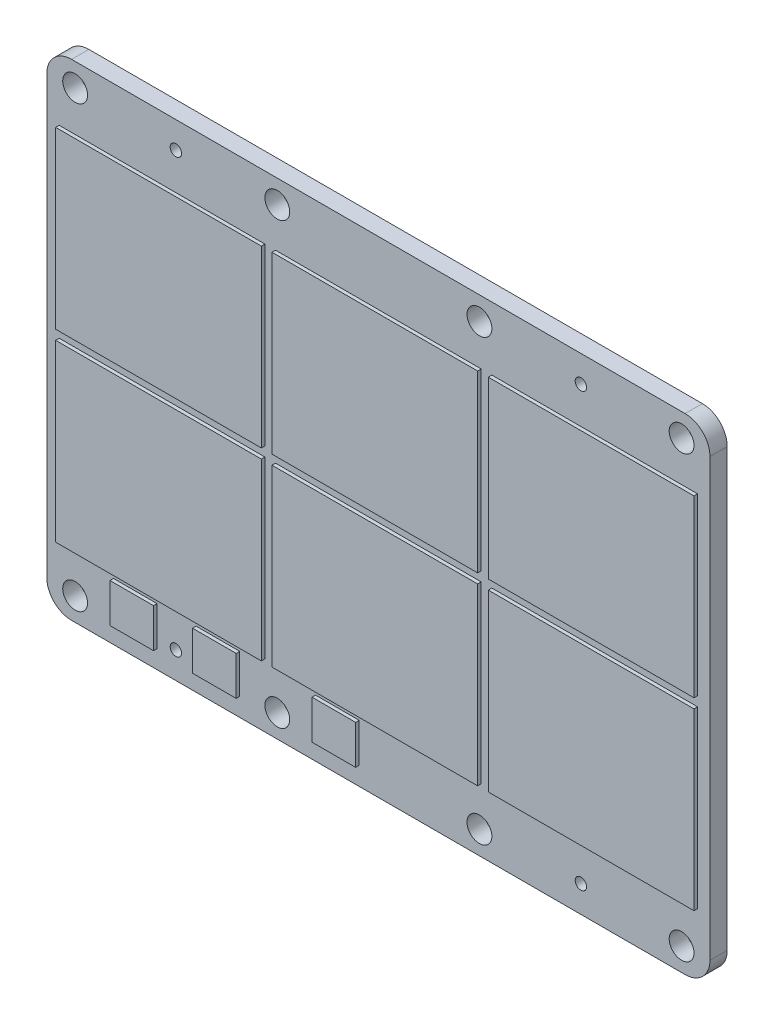
SolidWorks part; units mm, degrees
ref_plane "Front Plane" through (0, 0, 0) normal (0, 0, 1) x (1, 0, 0)
ref_plane "Top Plane" through (0, 0, 0) normal (0, 1, 0) x (1, 0, 0)
ref_plane "Right Plane" through (0, 0, 0) normal (1, 0, 0) x (0, 0, -1)
sketch "Sketch1" plane through (0, 0, 0) normal (0, 0, 1) x (1, 0, 0)
  line L1 (-93.5, 68.5) -> (93.5, 68.5)
  line L2 (-93.5, 68.5) -> (-93.5, -68.5)
  line L3 (-93.5, -68.5) -> (93.5, -68.5)
  line L4 (93.5, 68.5) -> (93.5, -68.5)
  line L5 (-93.5, 68.5) -> (93.5, -68.5) construction
  line L6 (-93.5, -68.5) -> (93.5, 68.5) construction
  point P0 (0, 0)
  dimension "D1" = 187
  dimension "D2" = 137
extrude "Boss-Extrude1" add sketch "Sketch1" along normal blind 4.87
hole_wizard "Ø7.0 (7) Diameter Hole1" positions "Sketch3" profile "Sketch2" hole size "Ø7.0" standard "ISO" end condition through all
sketch "Sketch3" plane through (0, 0, 4.87) normal (0, 0, 1) x (1, 0, 0)
  line L0 (-93.5, 68.5) -> (-93.5, -68.5) construction
  line L1 (0, 0) -> (-28.5, 0) construction
  point P0 (-28.5, 62)
  point P1 (-85.5, 62)
  point P3 (28.5, 62)
  point P9 (85.5, 62)
  point P19 (85.5, -62)
  point P20 (28.5, -62)
  point P21 (-85.5, -62)
  point P22 (-28.5, -62)
  dimension "D1" = 57
  dimension "D2" = 57
  dimension "D3" = 57
  dimension "D4" = 8
  dimension "D5" = 62
sketch "Sketch2" plane through (-28.5, 62, 4.87) normal (1, 0, 0) x (0, -1, 0)
  line L0 (0, 0) -> (0, 4.87)
  line L1 (0, 4.87) -> (3.5, 4.87)
  line L2 (3.5, 4.87) -> (3.5, 0)
  line L5 (3.5, 0) -> (0, 0)
  line L11 (0, -6.35) -> (0, 107.95) construction
  dimension "通孔孔直径" = 7
  dimension "通孔孔深度" = 4.87
hole_wizard "Ø3.2 (3.2) Diameter Hole1" positions "Sketch4" profile "Sketch5" hole size "Ø3.2" standard "ISO" end condition through all
sketch "Sketch4" plane through (0, 0, 4.87) normal (0, 0, 1) x (1, 0, 0)
  line L1 (0, 0) -> (30.398, 0) construction
  line L3 (-93.5, 68.5) -> (-93.5, -68.5) construction
  point P0 (-57.1, 61.02)
  point P2 (57.1, 60.975)
  point P4 (57.1, -60.975)
  point P6 (-57.1, -61.02)
  dimension "D1" = 121.95
  dimension "D2" = 122.04
  dimension "D3" = 36.4
  dimension "D4" = 114.2
sketch "Sketch5" plane through (-57.1, 61.02, 4.87) normal (1, 0, 0) x (0, -1, 0)
  line L0 (0, 0) -> (0, 4.87)
  line L1 (0, 4.87) -> (1.6, 4.87)
  line L2 (1.6, 4.87) -> (1.6, 0)
  line L5 (1.6, 0) -> (0, 0)
  line L11 (0, -6.35) -> (0, 107.95) construction
  dimension "通孔孔直径" = 3.2
  dimension "通孔孔深度" = 4.87
sketch "Sketch6" plane through (0, 0, 4.87) normal (0, 0, 1) x (1, 0, 0)
  line L1 (-90, 50.65) -> (-32, 50.65)
  line L2 (-90, 50.65) -> (-90, -50.65)
  line L3 (-90, -50.65) -> (-32, -50.65)
  line L4 (-32, 50.65) -> (-32, -50.65)
  line L5 (-32, 0) -> (0, 0) construction
  line L6 (-93.5, 68.5) -> (-93.5, -68.5) construction
  line L7 (-29, 50.65) -> (-29, -50.65)
  line L8 (-29, 50.65) -> (29, 50.65)
  line L9 (29, 50.65) -> (29, -50.65)
  line L10 (-29, -50.65) -> (29, -50.65)
  line L11 (32, 50.65) -> (32, -50.65)
  line L12 (32, 50.65) -> (90, 50.65)
  line L13 (90, 50.65) -> (90, -50.65)
  line L14 (32, -50.65) -> (90, -50.65)
  dimension "D1" = 101.3
  dimension "D2" = 58
  dimension "D3" = 3.5
  dimension "D5" = 3
  dimension "D4" = 3
extrude "Boss-Extrude2" add sketch "Sketch6" along normal blind 1
sketch "Sketch7" plane through (0, 0, 4.87) normal (0, 0, 1) x (1, 0, 0)
  line L0 (-93.5, -68.5) -> (93.5, -68.5) construction
  line L1 (-74.7, -52.35) -> (-62.4, -52.35)
  line L2 (-74.7, -52.35) -> (-74.7, -63.35)
  line L3 (-74.7, -63.35) -> (-62.4, -63.35)
  line L4 (-62.4, -52.35) -> (-62.4, -63.35)
  line L5 (-93.5, 68.5) -> (-93.5, -68.5) construction
  line L6 (-51.39, -52.35) -> (-51.39, -63.35)
  line L7 (-51.39, -52.35) -> (-39.09, -52.35)
  line L8 (-39.09, -52.35) -> (-39.09, -63.35)
  line L9 (-51.39, -63.35) -> (-39.09, -63.35)
  line L10 (-17.69, -52.35) -> (-17.69, -63.35)
  line L11 (-17.69, -63.35) -> (-5.39, -63.35)
  line L12 (-5.39, -52.35) -> (-5.39, -63.35)
  line L13 (-17.69, -52.35) -> (-5.39, -52.35)
  dimension "D1" = 12.3
  dimension "D2" = 11
  dimension "D3" = 5.15
  dimension "D4" = 18.8
  dimension "D6" = 11.01
  dimension "D8" = 21.4
  dimension "D5" = 2
  dimension "D7" = 2
extrude "Boss-Extrude3" add sketch "Sketch7" along normal blind 1
sketch "Sketch8" plane through (0, 0, 5.87) normal (0, 0, 1) x (1, 0, 0)
  line L1 (-101.7092, 1.35) -> (101.7092, 1.35)
  line L2 (-101.7092, 1.35) -> (-101.7092, -1.35)
  line L3 (-101.7092, -1.35) -> (101.7092, -1.35)
  line L4 (101.7092, 1.35) -> (101.7092, -1.35)
  line L5 (-101.7092, 1.35) -> (101.7092, -1.35) construction
  line L6 (-101.7092, -1.35) -> (101.7092, 1.35) construction
  point P0 (0, 0)
  dimension "D1" = 2.7
extrude "Cut-Extrude1" cut sketch "Sketch8" against normal up to surface (1 mm away) up to face at (-61, 0, 4.87)
fillet "Fillet1" radius 7 4 edges at (-93.5, -68.5, 2.435) (93.5, -68.5, 2.435) (93.5, 68.5, 2.435) (-93.5, 68.5, 2.435)
